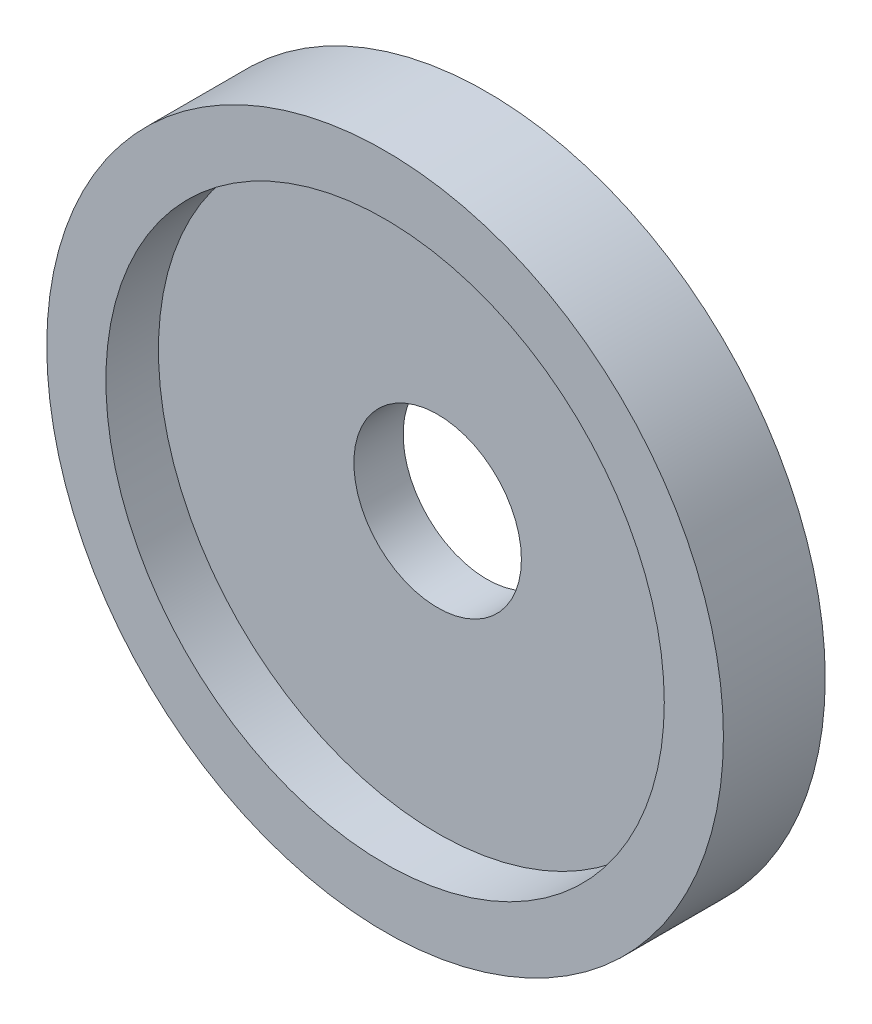
from build123d import *

# Parameters (mm, degrees)
SKETCH1_R           = 103
SKETCH1_R_2         = 25.5
BOSS_EXTRUDE1_DEPTH = 15
SKETCH2_R           = 103
SKETCH2_R_2         = 85
BOSS_EXTRUDE2_DEPTH = 16


with BuildPart() as part:
    # Sketch1 → Boss-Extrude1 (new body)
    with BuildSketch(Plane.XY):
        Circle(SKETCH1_R)
        Circle(SKETCH1_R_2, mode=Mode.SUBTRACT)
    extrude(amount=BOSS_EXTRUDE1_DEPTH)

    # Sketch2 → Boss-Extrude2 (add)
    with BuildSketch(Plane.XY.offset(15)):
        Circle(SKETCH2_R)
        Circle(SKETCH2_R_2, mode=Mode.SUBTRACT)
    extrude(amount=BOSS_EXTRUDE2_DEPTH)


solid = part.part
